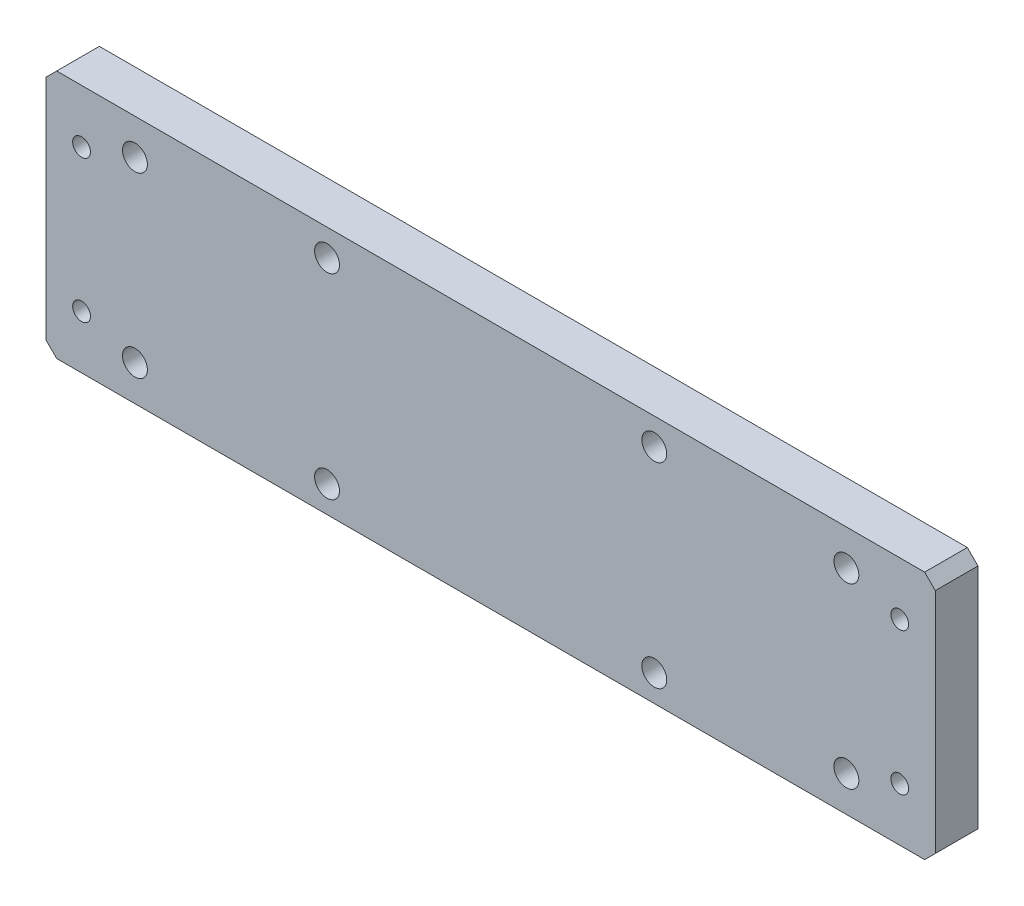
from build123d import *

# Parameters (mm, degrees)
SKETCH_1_W            = 250
SKETCH_1_H            = 70
EXTRUDE_1_DEPTH       = 12
CHAMFER_1_SIZE        = 3
HOLE_WIZARD_7_0_7_1_D = 7
HOLE_WIZARD_M6_1_D    = 5
HOLE_WIZARD_7_0_7_2_D = 7


with BuildPart() as part:
    # 草图1 → 凸台-拉伸1 (new body)
    with BuildSketch(Plane.XY):
        Rectangle(SKETCH_1_W, SKETCH_1_H)
    extrude(amount=EXTRUDE_1_DEPTH)

    # 倒角1
    chamfer_1_edges = [part.edges().sort_by_distance(p)[0] for p in [
        (125, -35, 6),
        (-125, -35, 6),
        (-125, 35, 6),
        (125, 35, 6),
    ]]
    chamfer(chamfer_1_edges, length=CHAMFER_1_SIZE)

    # Ø7.0 (7) 直径孔1 (through all)
    with Locations(Plane(origin=(0, 0, 0), x_dir=(-1, 0, 0), z_dir=(0, 0, -1))):
        with Locations((100, -25), (100, 25), (-100, 25), (-100, -25)):
            Hole(HOLE_WIZARD_7_0_7_1_D / 2)

    # M6 螺纹孔1 (through all)
    with Locations(Plane(origin=(0, 0, 0), x_dir=(-1, 0, 0), z_dir=(0, 0, -1))):
        with Locations((115, -20), (115, 20), (-115, 20), (-115, -20)):
            Hole(HOLE_WIZARD_M6_1_D / 2)

    # Ø7.0 (7) 直径孔2 (through all)
    with Locations(Plane(origin=(0, 0, 0), x_dir=(-1, 0, 0), z_dir=(0, 0, -1))):
        with Locations((46, 27.5), (46, -27.5), (-46, 27.5), (-46, -27.5)):
            Hole(HOLE_WIZARD_7_0_7_2_D / 2)


solid = part.part
